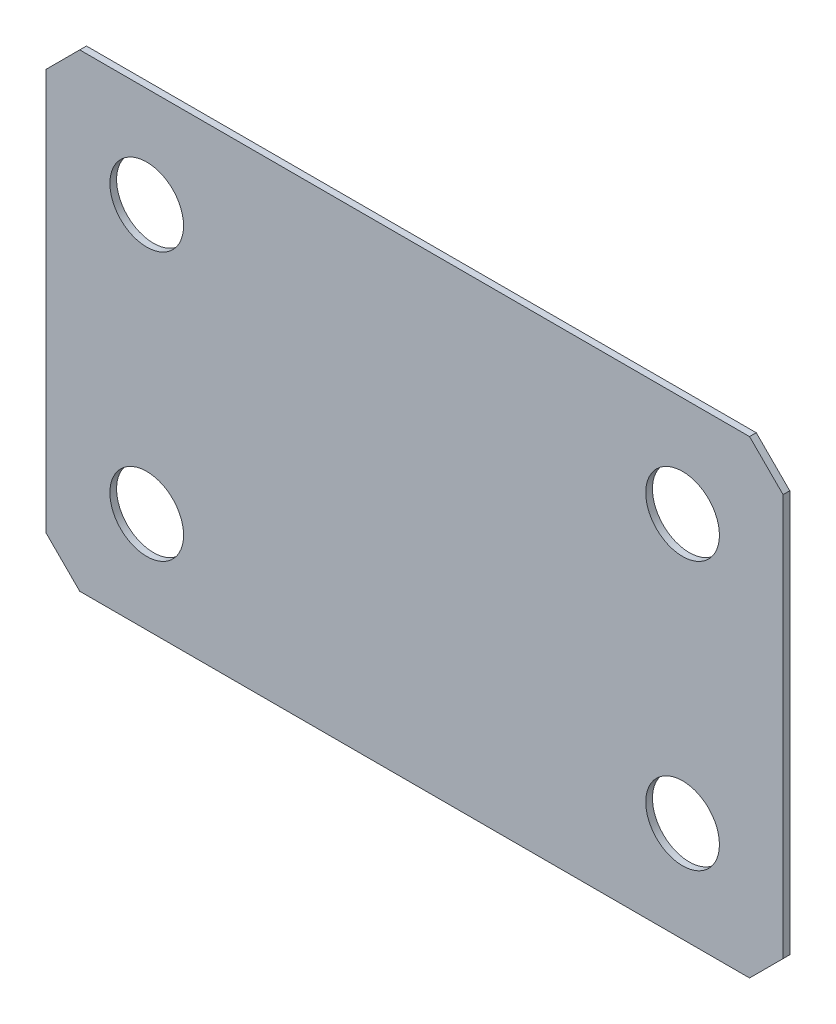
SolidWorks part; units mm, degrees
material "1023 carbon steel plate (SS)"
ref_plane "Front Plane" through (0, 0, 0) normal (0, 0, 1) x (1, 0, 0)
ref_plane "Top Plane" through (0, 0, 0) normal (0, 1, 0) x (1, 0, 0)
ref_plane "Right Plane" through (0, 0, 0) normal (1, 0, 0) x (0, 0, -1)
sketch "Sketch1" plane through (0, 0, 0) normal (0, 0, 1) x (1, 0, 0)
  line L1 (55, 35) -> (-55, 35)
  line L2 (55, 35) -> (55, -35)
  line L3 (55, -35) -> (-55, -35)
  line L4 (-55, 35) -> (-55, -35)
  line L5 (55, 35) -> (-55, -35) construction
  line L6 (55, -35) -> (-55, 35) construction
  point P0 (0, 0)
  dimension "D1" = 110
  dimension "D2" = 70
extrude "Boss-Extrude1" add sketch "Sketch1" along normal blind 1
sketch "Sketch2" plane through (0, 0, 1) normal (0, 0, 1) x (1, 0, 0)
  circle A0 centre (-40, 20) radius 5.5
  circle A1 centre (40, 20) radius 5.5
  circle A2 centre (-40, -20) radius 5.5
  circle A3 centre (40, -20) radius 5.5
  dimension "D3" = 20
  dimension "D4" = 40
  dimension "D5" = 11
  dimension "D1" = 80
  dimension "D2" = 40
extrude "Cut-Extrude1" cut sketch "Sketch2" against normal blind 1
chamfer "Chamfer1" distance 5 angle 45 4 edges at (-55, -35, 0.5) (55, -35, 0.5) (55, 35, 0.5) (-55, 35, 0.5)
